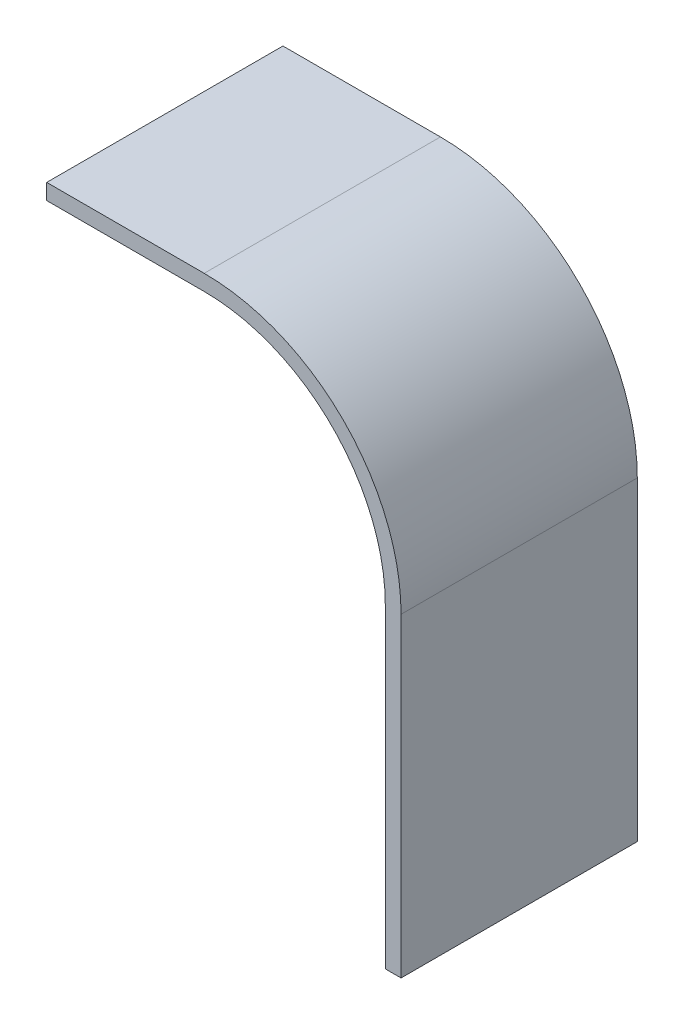
SolidWorks part; units mm, degrees
ref_plane "Front Plane" through (0, 0, 0) normal (0, 0, 1) x (1, 0, 0)
ref_plane "Top Plane" through (0, 0, 0) normal (0, 1, 0) x (1, 0, 0)
ref_plane "Right Plane" through (0, 0, 0) normal (1, 0, 0) x (0, 0, -1)
sketch "Sketch1" plane through (0, 0, 0) normal (0, 0, 1) x (1, 0, 0)
  line L0 (0, 0) -> (0, 40)
  line L1 (-10, 50) -> (-30, 50)
  arc A0 (0, 40) -> (-10, 50) centre (-10, 40) ccw
  point P6 (0, 50)
  dimension "D3" = 10
  dimension "D1" = 50
  dimension "D2" = 30
extrude "Extrude-Thin1" add sketch "Sketch1" along normal blind 2 thin
sketch "Sketch2" plane through (0, 0, 2) normal (0, 0, 1) x (1, 0, 0)
  line L0 (13, 0) -> (13, 40)
  line L1 (-10, 63) -> (-30, 63)
  line L2 (-30, 65) -> (-30, 63)
  line L3 (15, 0) -> (13, 0)
  line L6 (-10, 65) -> (-30, 65)
  line L7 (-30, 65) -> (-30, 50)
  line L8 (-30, 50) -> (-10, 50)
  line L9 (0, 40) -> (0, 0)
  line L10 (0, 0) -> (15, 0)
  line L11 (15, 0) -> (15, 40)
  line L12 (-10, 65) -> (-30, 65)
  line L17 (15, 0) -> (15, 40)
  arc A0 (13, 40) -> (-10, 63) centre (-10, 40) ccw
  arc A2 (0, 40) -> (-10, 50) centre (-10, 40) ccw
  arc A3 (15, 40) -> (-10, 65) centre (-10, 40) ccw
  arc A5 (15, 40) -> (-10, 65) centre (-10, 40) ccw
  dimension "D1" = 0
  dimension "D2" = 2
extrude "Boss-Extrude1" add sketch "Sketch2" along normal blind 28
sketch "Sketch3" plane through (0, 0, 2) normal (0, 0, 1) x (1, 0, 0)
  line L0 (-21.0353, 59.1763) -> (-21.0353, 52.8359) construction
  line L1 (-19.2839, 59.1763) -> (-19.2839, 52.8359)
  line L2 (-22.7867, 59.1763) -> (-22.7867, 52.8359)
  line L3 (3.8424, 12.1195) -> (8.5885, 12.1195) construction
  line L4 (3.8424, 13.6957) -> (8.5885, 13.6957)
  line L5 (3.8424, 10.5433) -> (8.5885, 10.5433)
  line L6 (3.8424, 35.9073) -> (8.5885, 35.9073) construction
  line L7 (3.8424, 37.7073) -> (8.5885, 37.7073)
  line L8 (3.8424, 34.1073) -> (8.5885, 34.1073)
  arc A0 (-19.2839, 59.1763) -> (-22.7867, 59.1763) centre (-21.0353, 59.1763) ccw
  arc A1 (-22.7867, 52.8359) -> (-19.2839, 52.8359) centre (-21.0353, 52.8359) ccw
  arc A2 (3.8424, 13.6957) -> (3.8424, 10.5433) centre (3.8424, 12.1195) ccw
  arc A3 (8.5885, 10.5433) -> (8.5885, 13.6957) centre (8.5885, 12.1195) ccw
  arc A4 (3.8424, 37.7073) -> (3.8424, 34.1073) centre (3.8424, 35.9073) ccw
  arc A5 (8.5885, 34.1073) -> (8.5885, 37.7073) centre (8.5885, 35.9073) ccw
  point P2 (-21.0353, 56.0061)
  point P7 (6.2154, 12.1195)
  point P14 (6.2154, 35.9073)
extrude "Cut-Extrude1" cut sketch "Sketch3" against normal blind 28
